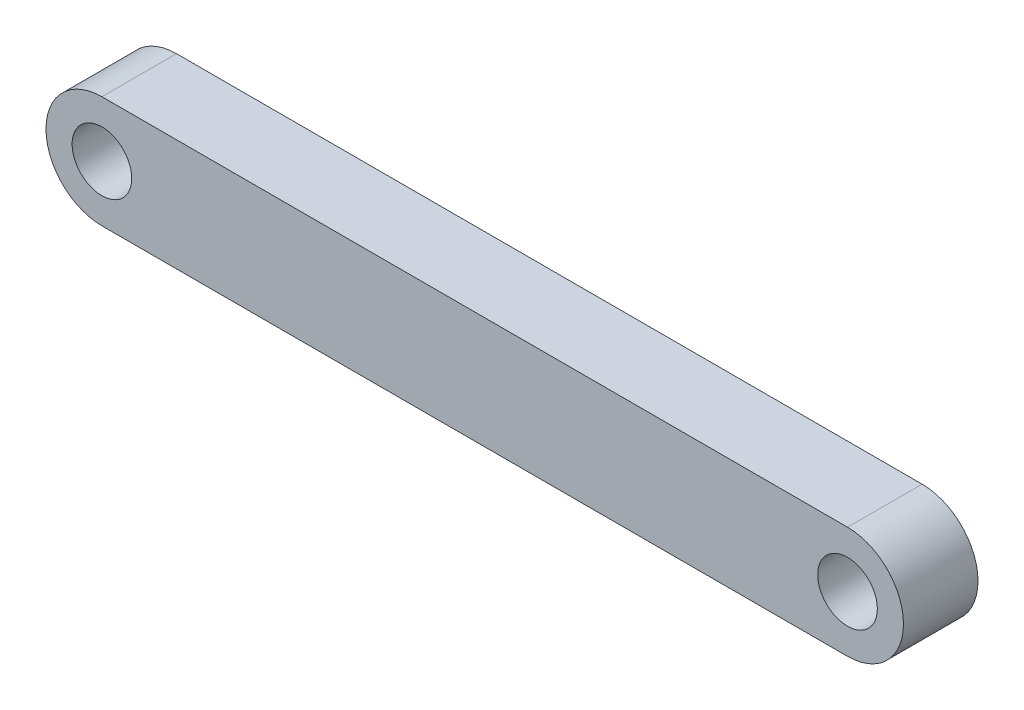
SolidWorks part; units mm, degrees
ref_plane "Front Plane" through (0, 0, 0) normal (0, 0, 1) x (1, 0, 0)
ref_plane "Top Plane" through (0, 0, 0) normal (0, 1, 0) x (1, 0, 0)
ref_plane "Right Plane" through (0, 0, 0) normal (1, 0, 0) x (0, 0, -1)
sketch "Sketch1" plane through (0, 0, 0) normal (0, 0, 1) x (1, 0, 0)
  line L0 (0, 7.5) -> (100, 7.5)
  line L1 (100, -7.5) -> (0, -7.5)
  circle A0 centre (0, 0) radius 4
  circle A1 centre (100, 0) radius 4
  arc A2 (0, 7.5) -> (0, -7.5) centre (0, 0) ccw
  arc A3 (100, -7.5) -> (100, 7.5) centre (100, 0) ccw
  dimension "D1" = 100
  dimension "D2" = 8
  dimension "D3" = 15
  dimension "D4" = 8
  dimension "D5" = 15
extrude "Boss-Extrude1" add sketch "Sketch1" along normal blind 10
